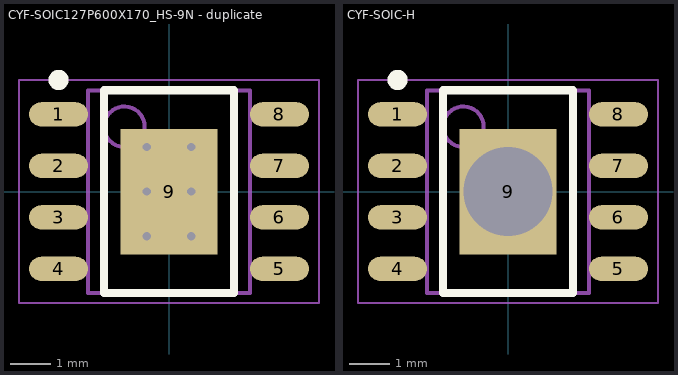
[diagram p0: the footprints below, top view; thin cyan lines are the x and y axes]
# Altium footprint library MISC82341-2.PcbLib: 2 footprints
Each footprint in its own frame and in the unit in brackets; x right, y up, seen from the top. Pads: shape width x height; smd on the part's side, far side on the other; paste and mask are expansions set on the pad; w line width, h text height; cw(c..) or ccw(c..) is an arc to the next point about the centre after c.

## CYF-SOIC127P600X170_HS-9N - duplicate [mm] "SOIC, 8-Leads, Body 4.90x3.90mm, Pitch 1.27mm, Thermal Pad 3.10x2.40mm, IPC Medium Density"
height 1.7
pads (9):
  oval 1.45x0.6 smd: 1(-2.725,1.905) 2(-2.725,0.635) 3(-2.725,-0.635) 4(-2.725,-1.905) 5(2.725,-1.905) 6(2.725,-0.635) 7(2.725,0.635) 8(2.725,1.905)
  rect 2.4x3.1 smd: 9(0,0)
via -0.55,1.1 diameter 0.5 hole 0.2
via 0.55,1.1 diameter 0.5 hole 0.2
via -0.55,0 diameter 0.5 hole 0.2
via 0.55,0 diameter 0.5 hole 0.2
via -0.55,-1.1 diameter 0.5 hole 0.2
via 0.55,-1.1 diameter 0.5 hole 0.2
Top Overlay:
  circle w0.25: c-2.725,2.755 r0.125
  lines w0.2: -1.6,-2.5 -1.6,2.5 1.6,2.5 1.6,-2.5 -1.6,-2.5
Mechanical 13:
  circle w0.1: c-1.1,1.6 r0.5
  lines w0.1: -2,-2.5 -2,2.5 2,2.5 2,-2.5 -2,-2.5
Mechanical 15:
  lines w0.05: -3.7,-2.75 -3.7,2.75 3.7,2.75 3.7,-2.75 -3.7,-2.75
  lines w0.1: -0.5,0 0.5,0 ; 0,-0.5 0,0.5
3D body: height 1.7, standoff 0.15, extent -2,-2.5 2,2.5

## CYF-SOIC-H [mm] "SOIC, 8-Leads, Body 4.90x3.90mm, Pitch 1.27mm, Thermal Pad 3.10x2.40mm, IPC Medium Density"
height 1.7
pads (9):
  oval 1.45x0.6 smd: 1(-2.725,1.905) 2(-2.725,0.635) 3(-2.725,-0.635) 4(-2.725,-1.905) 5(2.725,-1.905) 6(2.725,-0.635) 7(2.725,0.635) 8(2.725,1.905)
  rect 2.4x3.1 hole 2.2: 9(0,0)
Top Overlay:
  circle w0.25: c-2.725,2.755 r0.125
  lines w0.2: -1.6,-2.5 -1.6,2.5 1.6,2.5 1.6,-2.5 -1.6,-2.5
Mechanical 13:
  circle w0.1: c-1.1,1.6 r0.5
  lines w0.1: -2,-2.5 -2,2.5 2,2.5 2,-2.5 -2,-2.5
Mechanical 15:
  lines w0.05: -3.7,-2.75 -3.7,2.75 3.7,2.75 3.7,-2.75 -3.7,-2.75
  lines w0.1: -0.5,0 0.5,0 ; 0,-0.5 0,0.5
3D body: height 1.7, standoff 0.15, extent -2,-2.5 2,2.5